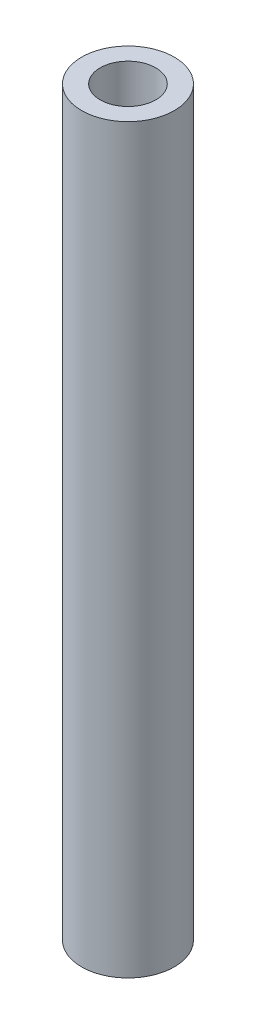
from build123d import *

# Parameters (mm, degrees)
SKETCH_1_R      = 2.5
SKETCH_1_R_2    = 1.5
EXTRUDE_1_DEPTH = 40


with BuildPart() as part:
    # 草图1 → 凸台-拉伸1 (new body)
    with BuildSketch(Plane(origin=(0, 0, 0), x_dir=(1, 0, 0), z_dir=(0, 1, 0))):
        with Locations(Location((0, 0, 0), (0, 0, 270))):
            Circle(SKETCH_1_R)
        with Locations(Location((0, 0, 0), (0, 0, 270))):
            Circle(SKETCH_1_R_2, mode=Mode.SUBTRACT)
    extrude(amount=EXTRUDE_1_DEPTH)


solid = part.part
